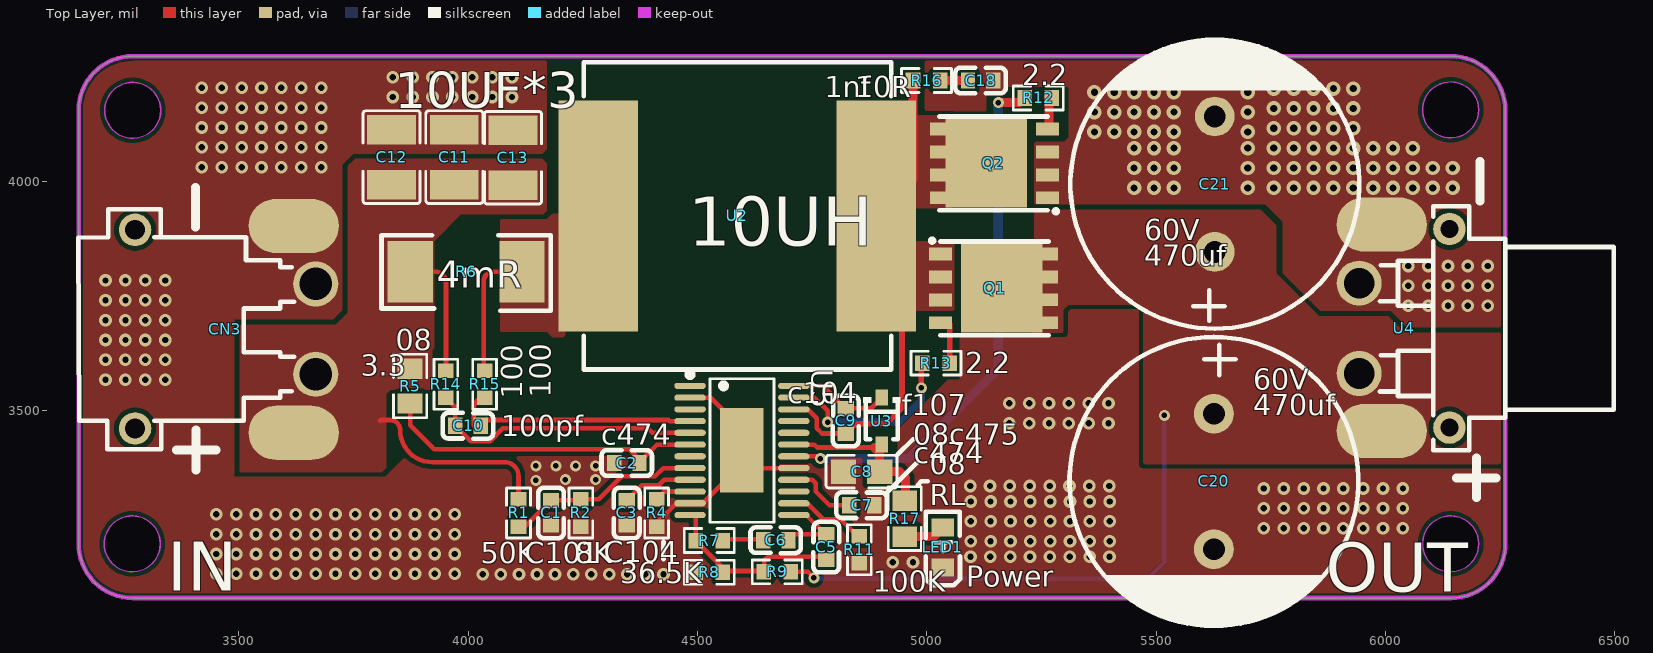
[diagram p0: Top Layer view]
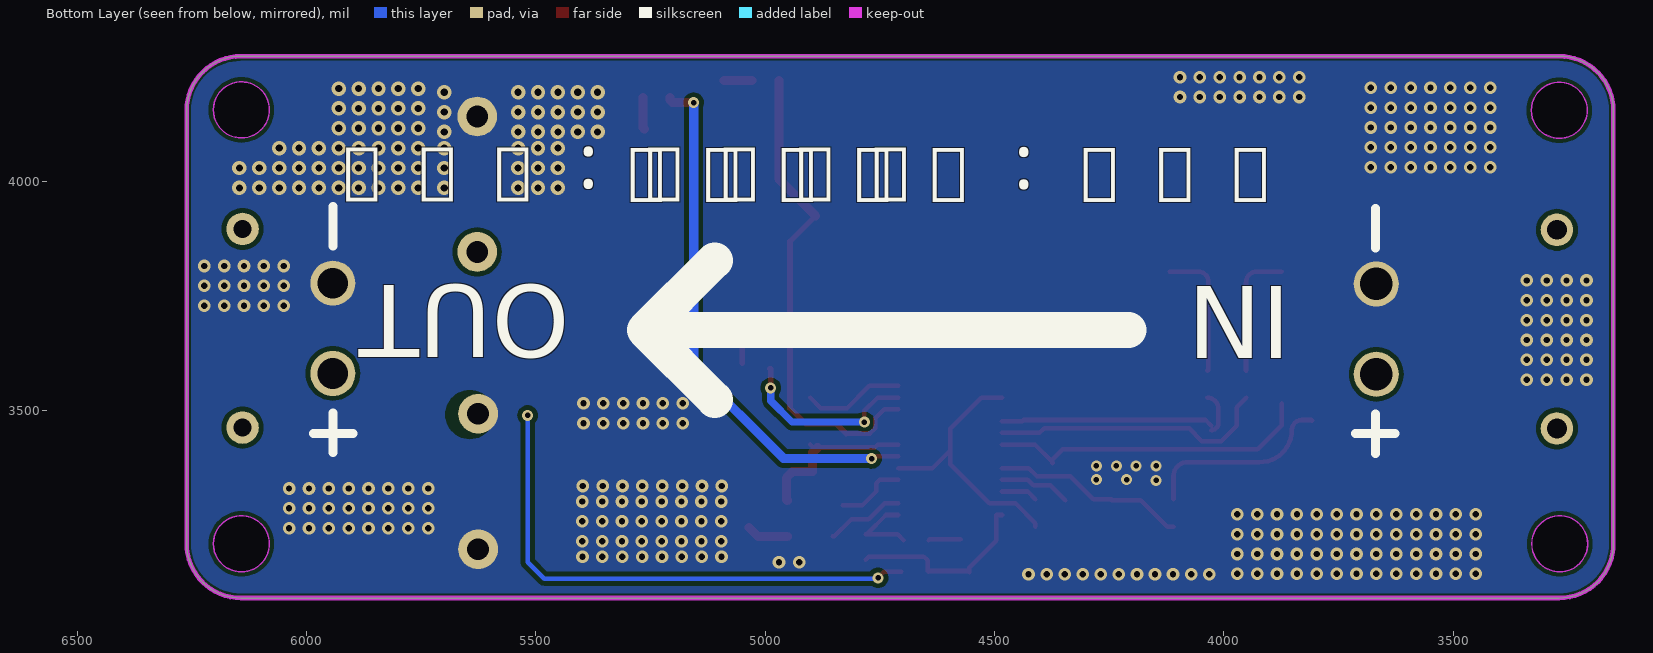
[diagram p1: Bottom Layer view, seen from below]
# Altium PCB MISC52028.pcbdoc
Units mil, origin at the board's own origin, x right, y up, seen from the top; angles counter-clockwise.
Board outline 3110.24 x 1181.1 mil, 2 copper layers (Top Layer, Bottom Layer), stack 62.206 mil thick; 38 components, 24 nets, 121 pads, 315 vias.

## Layer stack, top to bottom
Top Solder Mask Layer: solder mask 0.394, Dk 3.3
Top Layer: signal copper 1.379
Dielectric1: surface 59.449, FR4, Dk 4.5
Bottom Layer: signal copper 1.378
Bottom Solder Mask Layer: solder mask 0.394, Dk 3.3

## Board outline
3269.11,4273 ccw(c3269.11,4154.89) 3151,4154.89 3151,3210.01 ccw(c3269.11,3210.01) 3269.11,3091.9 6143.13,3091.9 ccw(c6143.13,3210.01) 6261.24,3210.01 6261.24,4154.89 ccw(c6143.13,4154.89) 6143.13,4273
cut-out: 3330.02,4155 cw(c3269,4155) 3207.98,4155 cw(c3269,4155)
cut-out: 6203.02,4156 cw(c6142,4156) 6080.98,4156 cw(c6142,4156)
cut-out: 6203.02,3210 cw(c6142,3210) 6080.98,3210 cw(c6142,3210)
cut-out: 3329.02,3210 cw(c3268,3210) 3206.98,3210 cw(c3268,3210)

## Design rules (kind name [scope] priority, off if disabled: settings)
BoardOutlineClearance copperThickness2oz_1 [All] p2 off: genericclearance=7.99 ignorepadtopadclearanceinfootprint=FALSE except(0: Arc-SplitContinuation Track-SplitContinuation SMDPad-SplitContinuation THPad-SplitContinuation Via-SplitContinuation Fill-SplitContinuation Region-SplitContinuation Poly-SplitContinuation Text-SplitContinuation Hole-SplitContinuation; 5.98: SMDPad-CutoutEdge THPad-CutoutEdge Via-CutoutEdge Fill-CutoutEdge Region-CutoutEdge Text-CutoutEdge Hole-CutoutEdge; 10: Poly-OutlineEdge Poly-CutoutEdge; 11.81: Arc-OutlineEdge Track-OutlineEdge SMDPad-OutlineEdge THPad-OutlineEdge Via-OutlineEdge Fill-OutlineEdge Region-OutlineEdge Text-OutlineEdge Hole-OutlineEdge Arc-CutoutEdge Track-CutoutEdge)
BoardOutlineClearance Plane_innerPlane_1 [All] p4 off: genericclearance=4.02 ignorepadtopadclearanceinfootprint=FALSE except(0: Arc-SplitContinuation Track-SplitContinuation SMDPad-SplitContinuation THPad-SplitContinuation Via-SplitContinuation Fill-SplitContinuation Region-SplitContinuation Poly-SplitContinuation Text-SplitContinuation Hole-SplitContinuation; 5.98: SMDPad-CutoutEdge THPad-CutoutEdge Via-CutoutEdge Fill-CutoutEdge Region-CutoutEdge Text-CutoutEdge Hole-CutoutEdge; 10: Poly-OutlineEdge Poly-CutoutEdge; 11.81: Arc-OutlineEdge Track-OutlineEdge SMDPad-OutlineEdge THPad-OutlineEdge Via-OutlineEdge Fill-OutlineEdge Region-OutlineEdge Text-OutlineEdge Hole-OutlineEdge Arc-CutoutEdge Track-CutoutEdge)
BoardOutlineClearance Copper_copperRegion_1 [All] p6 off: genericclearance=4.02 ignorepadtopadclearanceinfootprint=FALSE except(0: Arc-SplitContinuation Track-SplitContinuation SMDPad-SplitContinuation THPad-SplitContinuation Via-SplitContinuation Fill-SplitContinuation Region-SplitContinuation Poly-SplitContinuation Text-SplitContinuation Hole-SplitContinuation; 5.98: SMDPad-CutoutEdge THPad-CutoutEdge Via-CutoutEdge Fill-CutoutEdge Region-CutoutEdge Text-CutoutEdge Hole-CutoutEdge; 10: Poly-OutlineEdge Poly-CutoutEdge; 11.81: Arc-OutlineEdge Track-OutlineEdge SMDPad-OutlineEdge THPad-OutlineEdge Via-OutlineEdge Fill-OutlineEdge Region-OutlineEdge Text-OutlineEdge Hole-OutlineEdge Arc-CutoutEdge Track-CutoutEdge)
BoardOutlineClearance Copper_全直连_1 [All] p8 off: genericclearance=4.02 ignorepadtopadclearanceinfootprint=FALSE except(0: Arc-SplitContinuation Track-SplitContinuation SMDPad-SplitContinuation THPad-SplitContinuation Via-SplitContinuation Fill-SplitContinuation Region-SplitContinuation Poly-SplitContinuation Text-SplitContinuation Hole-SplitContinuation; 5.98: SMDPad-CutoutEdge THPad-CutoutEdge Via-CutoutEdge Fill-CutoutEdge Region-CutoutEdge Text-CutoutEdge Hole-CutoutEdge; 10: Poly-OutlineEdge Poly-CutoutEdge; 11.81: Arc-OutlineEdge Track-OutlineEdge SMDPad-OutlineEdge THPad-OutlineEdge Via-OutlineEdge Fill-OutlineEdge Region-OutlineEdge Text-OutlineEdge Hole-OutlineEdge Arc-CutoutEdge Track-CutoutEdge)
BoardOutlineClearance Copper_copperRegion2_1 [All] p10 off: genericclearance=4.02 ignorepadtopadclearanceinfootprint=FALSE except(0: Arc-SplitContinuation Track-SplitContinuation SMDPad-SplitContinuation THPad-SplitContinuation Via-SplitContinuation Fill-SplitContinuation Region-SplitContinuation Poly-SplitContinuation Text-SplitContinuation Hole-SplitContinuation; 5.98: SMDPad-CutoutEdge THPad-CutoutEdge Via-CutoutEdge Fill-CutoutEdge Region-CutoutEdge Text-CutoutEdge Hole-CutoutEdge; 10: Poly-OutlineEdge Poly-CutoutEdge; 11.81: Arc-OutlineEdge Track-OutlineEdge SMDPad-OutlineEdge THPad-OutlineEdge Via-OutlineEdge Fill-OutlineEdge Region-OutlineEdge Text-OutlineEdge Hole-OutlineEdge Arc-CutoutEdge Track-CutoutEdge)
BoardOutlineClearance copperThickness1oz_1 [All] p12: genericclearance=4.02 ignorepadtopadclearanceinfootprint=FALSE except(0: Arc-SplitContinuation Track-SplitContinuation SMDPad-SplitContinuation THPad-SplitContinuation Via-SplitContinuation Fill-SplitContinuation Region-SplitContinuation Poly-SplitContinuation Text-SplitContinuation Hole-SplitContinuation; 5.98: SMDPad-CutoutEdge THPad-CutoutEdge Via-CutoutEdge Fill-CutoutEdge Region-CutoutEdge Text-CutoutEdge Hole-CutoutEdge; 10: Poly-OutlineEdge Poly-CutoutEdge; 11.81: Arc-OutlineEdge Track-OutlineEdge SMDPad-OutlineEdge THPad-OutlineEdge Via-OutlineEdge Fill-OutlineEdge Region-OutlineEdge Text-OutlineEdge Hole-OutlineEdge Arc-CutoutEdge Track-CutoutEdge)
Clearance copperThickness2oz [All] p1 off: gap=7.99 ignorepadtopadclearanceinfootprint=FALSE except(5.98: SMDPad-Track SMDPad-SMDPad THPad-Track SMDPad-THPad THPad-THPad Track-Via SMDPad-Via THPad-Via Via-Via Fill-Track Region-Track Fill-SMDPad Region-SMDPad Fill-THPad Region-THPad Fill-Via Region-Via Fill-Fill Fill-Region Region-Region Arc-Track Arc-SMDPad Arc-THPad Arc-Via Fill-Arc Region-Arc Arc-Arc Text-Track SMDPad-Text Text-THPad Text-Via Fill-Text Region-Text Arc-Text Text-Text Hole-Track Hole-SMDPad Hole-THPad Hole-Via Fill-Hole Region-Hole Hole-Arc Hole-Text; 10: Poly-Track Poly-SMDPad Poly-THPad Poly-Via Poly-Fill Poly-Region Poly-Poly Poly-Arc Poly-Text Poly-Hole)
Clearance Plane_innerPlane [All] p3 off: gap=4.02 ignorepadtopadclearanceinfootprint=FALSE except(5.98: SMDPad-Track SMDPad-SMDPad THPad-Track SMDPad-THPad THPad-THPad Track-Via SMDPad-Via THPad-Via Via-Via Fill-Track Region-Track Fill-SMDPad Region-SMDPad Fill-THPad Region-THPad Fill-Via Region-Via Fill-Fill Fill-Region Region-Region Arc-Track Arc-SMDPad Arc-THPad Arc-Via Fill-Arc Region-Arc Arc-Arc Text-Track SMDPad-Text Text-THPad Text-Via Fill-Text Region-Text Arc-Text Text-Text Hole-Track Hole-SMDPad Hole-THPad Hole-Via Fill-Hole Region-Hole Hole-Arc Hole-Text; 10: Poly-Track Poly-SMDPad Poly-THPad Poly-Via Poly-Fill Poly-Region Poly-Poly Poly-Arc Poly-Text Poly-Hole)
Clearance Copper_copperRegion [All] p5 off: gap=4.02 ignorepadtopadclearanceinfootprint=FALSE except(5.98: SMDPad-Track SMDPad-SMDPad THPad-Track SMDPad-THPad THPad-THPad Track-Via SMDPad-Via THPad-Via Via-Via Fill-Track Region-Track Fill-SMDPad Region-SMDPad Fill-THPad Region-THPad Fill-Via Region-Via Fill-Fill Fill-Region Region-Region Arc-Track Arc-SMDPad Arc-THPad Arc-Via Fill-Arc Region-Arc Arc-Arc Text-Track SMDPad-Text Text-THPad Text-Via Fill-Text Region-Text Arc-Text Text-Text Hole-Track Hole-SMDPad Hole-THPad Hole-Via Fill-Hole Region-Hole Hole-Arc Hole-Text; 10: Poly-Track Poly-SMDPad Poly-THPad Poly-Via Poly-Fill Poly-Region Poly-Poly Poly-Arc Poly-Text Poly-Hole)
Clearance Copper_全直连 [All] p7 off: gap=4.02 ignorepadtopadclearanceinfootprint=FALSE except(5.98: SMDPad-Track SMDPad-SMDPad THPad-Track SMDPad-THPad THPad-THPad Track-Via SMDPad-Via THPad-Via Via-Via Fill-Track Region-Track Fill-SMDPad Region-SMDPad Fill-THPad Region-THPad Fill-Via Region-Via Fill-Fill Fill-Region Region-Region Arc-Track Arc-SMDPad Arc-THPad Arc-Via Fill-Arc Region-Arc Arc-Arc Text-Track SMDPad-Text Text-THPad Text-Via Fill-Text Region-Text Arc-Text Text-Text Hole-Track Hole-SMDPad Hole-THPad Hole-Via Fill-Hole Region-Hole Hole-Arc Hole-Text; 10: Poly-Track Poly-SMDPad Poly-THPad Poly-Via Poly-Fill Poly-Region Poly-Poly Poly-Arc Poly-Text Poly-Hole)
Clearance Copper_copperRegion2 [All] p9 off: gap=4.02 ignorepadtopadclearanceinfootprint=FALSE except(5.98: SMDPad-Track SMDPad-SMDPad THPad-Track SMDPad-THPad THPad-THPad Track-Via SMDPad-Via THPad-Via Via-Via Fill-Track Region-Track Fill-SMDPad Region-SMDPad Fill-THPad Region-THPad Fill-Via Region-Via Fill-Fill Fill-Region Region-Region Arc-Track Arc-SMDPad Arc-THPad Arc-Via Fill-Arc Region-Arc Arc-Arc Text-Track SMDPad-Text Text-THPad Text-Via Fill-Text Region-Text Arc-Text Text-Text Hole-Track Hole-SMDPad Hole-THPad Hole-Via Fill-Hole Region-Hole Hole-Arc Hole-Text; 10: Poly-Track Poly-SMDPad Poly-THPad Poly-Via Poly-Fill Poly-Region Poly-Poly Poly-Arc Poly-Text Poly-Hole)
Clearance copperThickness1oz [All] p11: gap=4.02 ignorepadtopadclearanceinfootprint=FALSE except(5.98: SMDPad-Track SMDPad-SMDPad THPad-Track SMDPad-THPad THPad-THPad Track-Via SMDPad-Via THPad-Via Via-Via Fill-Track Region-Track Fill-SMDPad Region-SMDPad Fill-THPad Region-THPad Fill-Via Region-Via Fill-Fill Fill-Region Region-Region Arc-Track Arc-SMDPad Arc-THPad Arc-Via Fill-Arc Region-Arc Arc-Arc Text-Track SMDPad-Text Text-THPad Text-Via Fill-Text Region-Text Arc-Text Text-Text Hole-Track Hole-SMDPad Hole-THPad Hole-Via Fill-Hole Region-Hole Hole-Arc Hole-Text; 10: Poly-Track Poly-SMDPad Poly-THPad Poly-Via Poly-Fill Poly-Region Poly-Poly Poly-Arc Poly-Text Poly-Hole)
DiffPairsRouting differentialPair [All] p1: maxlimit=6 minlimit=6 mostfreqgap=6 toplayer_minwidth=5 toplayer_prefwidth=10 toplayer_maxwidth=100 toplayer_mingap=6 toplayer_prefgap=6 toplayer_maxgap=6 bottomlayer_minwidth=5 bottomlayer_prefwidth=10 bottomlayer_maxwidth=100 bottomlayer_mingap=6 bottomlayer_prefgap=6 bottomlayer_maxgap=6 maxuncoupledlength=10
HoleToHoleClearance otherClearance [All] p1: gap=11.8 allowstackedmicrovias=TRUE
Length netLength [All] p1: minlimit=0 maxlimit=0
PasteMaskExpansion pasteMaskExpansion [All] p1: expansion=0
PlaneConnect innerPlane [All] p1: planeconnectstyle=Relief reliefexpansion=20 reliefentries=4 reliefconductorwidth=10 reliefairgap=10
PolygonConnect 全直连 [All] p1 off: connectstyle=Direct reliefconductorwidth=10 reliefentries=4 polygonreliefangle="90 Angle" airgapwidth=10 via.connectstyle=Relief via.reliefconductorwidth=10 via.reliefentries=4 via.polygonreliefangle="90 Angle" via.airgapwidth=10
PolygonConnect copperRegion2 [All] p2 off: connectstyle=Relief reliefconductorwidth=10 reliefentries=4 polygonreliefangle="90 Angle" airgapwidth=10 via.connectstyle=Relief via.reliefconductorwidth=10 via.reliefentries=4 via.polygonreliefangle="90 Angle" via.airgapwidth=10
PolygonConnect copperRegion [All] p3: connectstyle=Relief reliefconductorwidth=10 reliefentries=4 polygonreliefangle="90 Angle" airgapwidth=10 via.connectstyle=Relief via.reliefconductorwidth=10 via.reliefentries=4 via.polygonreliefangle="90 Angle" via.airgapwidth=10
RoutingVias viaSize [All] p1: holewidth=12.01 width=24.02 viastyle="Through Hole" minholewidth=11.81 minwidth=19.68 maxholewidth=248.03 maxwidth=393.7
SolderMaskExpansion solderMaskExpansion [IsVia] p1: expansion=-1000 istentingtop=TRUE
SolderMaskExpansion solderMaskExpansion [All] p2: expansion=2.01 istentingtop=FALSE
Width copperThickness2oz_2 [All] p1 off: maxlimit=100 minlimit=8 preferedwidth=10
Width copperThickness1oz_2 [All] p2: maxlimit=100 minlimit=5 preferedwidth=10

## Components (designator, comment, footprint, x,y, rotation, side; value= is the part's Value field where it differs from the comment)
C1 "100pF" C0603 4181,3277.61 r90 top
C2 "470nF" C0603 4346.2,3386.16 r0 top
C3 "100nF" C0603 4346,3277.61 r90 top
C5 "300pF" C0603 4781,3203 r90 top
C6 "34nF" C0603 4671,3217.84 r0 top
C7 "470nF" C0603 4858.16,3294 r0 top
C8 "4.7uf" C0805 4857.86,3367.46 r180 top
C9 "100nF" C0603 4823.65,3478 r90 top
C10 "100pf" C0603 4000,3467.3 r0 top
C11 "10uF" C1210 3970.17,4053 r270 top
C12 "10uF" C1210 3833.24,4053 r270 top
C13 "10uF" C1210 4097.93,4051.73 r270 top
C18 "100nF" C0603 5117.5,4220 r0 top
C20 "470uF" CAP-TH_BD16.0-P7.50-D1.2-FD 5626,3346 r270 top
C21 "470uF" CAP-TH_BD16.0-P7.50-D1.2-FD 5628,3994 r90 top
CN3 "XT30PW-M" CONN-TH_XT30PW-M 3471,3678 r270 top
LED1 "" LED_0805 5035.33,3204 r90 top
Q1 "CSD18540Q5B" VSON-CLIP-8_L5.0-W6.0-P1.27-BL 5147.91,3766.73 r270 top
Q2 "CSD18540Q5B" VSON-CLIP-8_L5.0-W6.0-P1.27-BL 5145.16,4039.22 r90 top
R1 "50K" R0603 4110,3277.31 r90 top
R2 "8K" R0603 4246,3277.31 r90 top
R4 "36.5K" R0603 4411,3277.31 r90 top
R5 "3.3" R0805_NEW 3873.84,3554 r90 top
R6 "4mΩ" RES-SMD_L6.4-W3.2-1 3995.89,3803 r0 top
R7 "40.53K" R0603 4526,3217.13 r0 top
R8 "1.6K" R0603 4526,3148 r0 top
R9 "30K" R0603 4673.84,3148.98 r0 top
R11 "100K" R0603 4852.97,3197.04 r90 top
R12 "2.2" R0603 5243.24,4182 r0 top
R13 "10K" R0603 5020,3604 r0 top
R14 "100" R0603 3951.66,3558 r90 top
R15 "100" R0603 4036,3558 r90 top
R16 "10K" R0603 4999.63,4220 r0 top
R17 "10K" R0805 4952,3265 r90 top
U2 "10uH" IND-SMD_L17.0-W17.0_YSPIA1770-100M 4587.2,3925 r0 top
U3 "FR107WS" SOD-323_L1.6-W1.3-LS2.7-RD 4902,3477.7 r270 top
U4 "XT30PW-F" CONN-TH_XT30PW-F-1 6041,3679.85 r90 top
U5 "LM5122ZAPWPR" HTSSOP-24_L7.8-W4.4-P0.65-LS6.4-BL-EP-3 4597.03,3413.55 r270 top

## Footprints (in the part's own frame and the unit in brackets; to place one, negate y for a bottom-side part, rotate by r counter-clockwise, add the part's x,y. Pads: shape width x height; smd on the part's side, far side on the other; paste and mask are expansions set on the pad)
C0603 [mm]
  rect 0.8x0.9 smd: 1(-0.7,0) 2(0.7,0)
  silkscreen extent -1.41,-0.71 1.39,0.72
C0805 [mm]
  rect 1.41x1.35 smd paste-100 mask+0.051: 1(-1,0) 2(1,0)
  silkscreen extent -1.96,-0.9 1.96,0.9
C1210 [mm]
  rect 1.635x2.7 smd paste-100 mask+0.051: 1(-1.517,0) 2(1.517,0)
  silkscreen extent -2.56,-1.58 2.56,1.58
CAP-TH_BD16.0-P7.50-D1.2-FD [mm]
  round 2.2 hole 1.2: 1(-3.75,0) 2(3.75,0)
  silkscreen extent -8,-8 8,8
CONN-TH_XT30PW-F-1 [mm]
  round 2.5 hole 1.7 copper offset 0,0: 1(-2.5,2.5) 2(2.5,2.5)
  round 1.8 hole 1 copper offset 0,0: 3(5.5,-2.5) 4(-5.5,-2.5)
  silkscreen extent -6.75,-11.6 6.75,1.35
CONN-TH_XT30PW-M [mm]
  round 2.5 hole 1.8: 1(-2.5,5) 2(2.5,5)
  round 1.8 hole 1.1: 3(5.5,-5) 4(-5.5,-5)
  silkscreen extent -6.65,-8.15 6.65,3.81
HTSSOP-24_L7.8-W4.4-P0.65-LS6.4-BL-EP-3 [mm]
  oval 0.343x1.747 smd: 1(-3.575,-2.873) 2(-2.925,-2.873) 3(-2.275,-2.873) 4(-1.625,-2.873) 5(-0.975,-2.873) 6(-0.325,-2.873) 7(0.325,-2.873) 8(0.975,-2.873) 9(1.625,-2.873) 10(2.275,-2.873) 11(2.925,-2.873) 12(3.575,-2.873) 13(3.575,2.873) 14(2.925,2.873) 15(2.275,2.873) 16(1.625,2.873) 17(0.975,2.873) 18(0.325,2.873) 19(-0.325,2.873) 20(-0.975,2.873) 21(-1.625,2.873) 22(-2.275,2.873) 23(-2.925,2.873) 24(-3.575,2.873)
  rect 4.68x2.4 smd: 25(0,0)
  silkscreen extent -4.35,-3.02 3.98,1.77
IND-SMD_L17.0-W17.0_YSPIA1770-100M [mm]
  rect 4.4x12.8 smd paste+0 mask+0.05: 1(-7.7,0) 2(7.7,0)
  silkscreen extent -8.51,-8.51 8.51,8.51
LED_0805 [mm]
  rect 1x1.25 smd paste+0 mask+0.051: 1(-1.15,0.005) 2(1.05,0.005)
  silkscreen extent -2.15,-0.94 1.93,0.97
R0603 [mil]
  rect 31.75x34.02 smd paste-3937.01 mask+2: 1(-29.66,0) 2(29.66,0)
  silkscreen extent -55,-26 55,26
R0805 [mm]
  rect 1.133x1.377 smd paste-100 mask+0.051: 1(-1,0) 2(1,0)
  silkscreen extent -1.76,-0.92 1.76,0.92
R0805_NEW [mil]
  rect 44.59x54.21 smd paste-3937.01 mask+2: 1(-38.04,0) 2(38.04,0)
  silkscreen extent -69,-36 69,36
RES-SMD_L6.4-W3.2-1 [mm]
  rect 2.5x3.4 smd: 1(-3.1,0) 2(3.1,0)
  silkscreen extent -4.69,-2.16 4.69,2.03
SOD-323_L1.6-W1.3-LS2.7-RD [mm]
  rect 0.9x0.7 smd paste+0 mask+0.05: 1(-1.3,0) 2(1.3,0)
  silkscreen extent -1.32,-1.02 1.02,1.02
VSON-CLIP-8_L5.0-W6.0-P1.27-BL [mm]
  rect 0.7x1.27 smd paste-100 mask+0.051: 1(-1.904,-3) 2(-0.636,-3) 3(0.636,-3) 4(1.906,-3)
  rect 0.7x1 smd paste-100 mask+0.051: 5(1.904,3) 6(0.634,3) 7(-0.636,3) 8(-1.906,3)
  rect 4.9x4.5 smd paste-100 mask+0.051: 8(-0.001,0.39)
  silkscreen extent -2.75,-3.57 2.6,3

## Free pads (board coordinates)
  oval 196.85x118.11 smd: 1(3620,3451.98) 1(3620,3903) 1(5991.79,3456) 1(5991.79,3906)

## Via types
v1: diameter 27.56, hole 13.8, Top Layer to Bottom Layer, 229 vias
v2: diameter 31.5, hole 15.7, Top Layer to Bottom Layer, 73 vias
v3: diameter 24.02, hole 12, Top Layer to Bottom Layer, 13 vias

## Nets (pads, with @x,y where several pads share a name; then routed paths per layer and width w, separated by ;. In a path a pad name is that pad's centre, name@x,y a point inside that pad or via, vN(x,y) a via of type N, cw(c..) or ccw(c..) an arc to the next point about the centre after c; other vN are vias at no path point)
$1N357: C1.2 R1.1 R2.2 U5.8 | length 426.7
  Top Layer w10: R1.1 4123.48,3247.65 C1.2 4244.2,3305.17 R2.2 4284.97,3306.97 4335.46,3357.46 4407.46,3357.46 4425.16,3375.16 U5.8
$1N466: C2.2 R5.1 U5.6 | length 710.5
  Top Layer w10: R5.1 3873.84,3468.16 3926,3416 4351.59,3416 C2.2@4376.61,3390.98 ; C2.2 4373.76,3388.13 C2.2@4376.61,3390.98 ; U5.6 4411.97,3426.34 C2.2@4376.61,3390.98
$1N636: C3.2 U5.9 | length 156.3
  Top Layer w10: C3.2 4378.83,3338 4416,3338 4427.57,3349.57 U5.9
$1N687: R4.2 U5.10 | length 80
  Top Layer w10: R4.2 4428.01,3323.98 U5.10
$1N1291: C6.1 R7.2 | length 70.3
  Top Layer w10: 4574,3220 4641.28,3220 C6.1
$1N1304: C5.2 C6.2 U5.13 | length 174.1
  Top Layer w10: C6.2 4711.28,3230.56 C5.2@4779.03,3230.56 ; U5.13 4736.79,3272.8 C5.2@4779.03,3230.56 ; C5.2 C5.2@4779.03,3230.56
$1N1428: C5.1 R7.1 R8.2 R9.1 U5.12 | length 420.1
  Top Layer w10: U5.12 4496.34,3272.8 R7.1 4555.66,3157.81 R8.2 4558.46,3150.8 R9.1@4646,3150.8 ; R9.1 R9.1@4646,3150.8 ; C5.1 4774.44,3182 4654,3182 4646,3174 R9.1@4646,3150.8
$1N1901: C9.2 U3.1 U5.24 | length 221.7
  Top Layer w10: U5.24 4772.94,3554.3 4821.68,3505.56 C9.2 4878.69,3505.56 U3.1
$1N2307: C7.1 U5.16 | length 154
  Top Layer w10: U5.16 4750.43,3349.57 4758,3342 4758,3324 4788,3294 C7.1
$1N2318: R11.2 U5.14 | length 172.5
  Top Layer w10: U5.14 4739.61,3298.39 4774,3264 4812,3264 4849.3,3226.7 R11.2
$1N3000: C9.1 Q1.1 Q1.2 Q1.3 Q2.5 Q2.6 Q2.7 Q2.8 R16.1 U2.2 U5.22 | length 1063.6
  Top Layer w10: U5.22 4740.88,3503.12 4760,3484 4760,3462 4771.56,3450.44 C9.1
  Top Layer w12: C9.1 4845.21,3472 4912,3472 4946,3506 4946,3869.34 U2.2
  Top Layer w20: U2.2 4969.97,4004.63 R16.1
$1N3130: R12.1 U5.18 | length 1168.3
  Top Layer w10: U5.18 4763.25,3400.75 v3(4768,3396)
  Top Layer w20: v3(5156,4172) 5202,4172 5207.45,4177.45 R12.1@5207.45,4183
  Bottom Layer w20: v3(4768,3396) 4960,3396 5156,3592 v3(5156,4172)
$1N3135: Q2.4 R12.2 | length 70.2
  Top Layer w20: Q2.4 5266.77,4117.75 R12.2@5266.77,4183
$1N3140: R13.1 U5.23 | length 405.8
  Top Layer w10: U5.23 4755.29,3528.71 4784,3500 v3(4784,3475.57)
  Top Layer w11.81: v3(4988,3550) 4988,3592.01 R13.1@4990.34,3592.01
  Bottom Layer w15.75: v3(4784,3475.57) 4941.57,3475.57 4988,3522 v3(4988,3550)
$1N3174: Q1.4 R13.2 | length 105.6
  Top Layer w11.81: Q1.4 5046.31,3691.69 5049.66,3688.34 R13.2
$1N3562: C10.1 R14.1 U5.5 | length 610.7
  Top Layer w10: R14.1 3972.44,3507.56 C10.1 4005.74,3434 4048,3434 4076,3462 4392,3462 4402.06,3451.94 U5.5
$1N3570: C10.2 R15.1 U5.4 | length 555.7
  Top Layer w10: C10.2 4040.26,3480 4437.06,3480 4439.53,3477.53 U5.4 ; C10.2@4027.89,3458 cw(c4027.89,3473.89) 4012,3473.89 4012,3504.34 cw(c4036,3504.34) R15.1
$1N3575: R6.2 R15.2 U2.1 | length 291.4
  Top Layer w10: R15.2 cw(c4036,3589.66) 4034,3589.66 4034,3782 cw(c4055,3782) 4055,3803 R6.2
$1N5355: C18.1 R16.2 | length 60.6
  Top Layer w20: R16.2 C18.1
$1N5615: LED1.2 R17.1 | length 91.3
  Top Layer w19.68: R17.1 5015.42,3225.63 LED1.2
AGND: C1.1 C2.1 C3.1 C7.2 C8.2 C11.1 C12.1 C13.1 C18.2 C20.2 C21.2 CN3.1 LED1.1 pad.1@3620,3903 pad.1@5991.79,3906 Q2.1 Q2.2 Q2.3 R2.1 R4.1 R8.1 R11.1 U4.2 U5.2 U5.11 U5.17 U5.25 | length 594.1
  Top Layer w10: R4.1 4411,3255 4454.39,3298.39 U5.11 4511.53,3298.39 4597.03,3383.88 U5.25 ; U5.2 4529.29,3528.71 4597.03,3460.97 U5.25 ; U5.17 4635.42,3375.16 U5.25
  other v1: 4032.22,3144 4071.59,3144 4110.96,3144 4150.33,3144 4189.7,3144 4229.07,3144 4268.44,3144 4307.81,3144 4347.18,3144 4386.55,3144 4425.92,3144 3451.16,3144.56 3494.47,3144.56 3537.78,3144.56 3581.09,3144.56 3624.39,3144.56 3667.7,3144.56 3711.01,3144.56 3754.31,3144.56 3797.62,3144.56 3840.93,3144.56 3884.24,3144.56 3927.54,3144.56 3970.85,3144.56 4926,3170 4970,3170 5095.23,3182 5138.54,3182 5181.84,3182 5225.15,3182 5268.46,3182 5311.76,3182 5355.07,3182 5398.38,3182 3451.16,3187.86 3494.47,3187.86 3537.78,3187.86 3581.09,3187.86 3624.39,3187.86 3667.7,3187.86 3711.01,3187.86 3754.31,3187.86 3797.62,3187.86 3840.93,3187.86 3884.24,3187.86 3927.54,3187.86 3970.85,3187.86 5095.78,3215.61 5139.09,3215.61 5182.39,3215.61 5225.7,3215.61 5269.01,3215.61 5312.31,3215.61 5355.62,3215.61 5398.93,3215.61 3451.16,3231.17 3494.47,3231.17 3537.78,3231.17 3581.09,3231.17 3624.39,3231.17 3667.7,3231.17 3711.01,3231.17 3754.31,3231.17 3797.62,3231.17 3840.93,3231.17 3884.24,3231.17 3927.54,3231.17 3970.85,3231.17 5734.85,3244 5778.16,3244 5821.46,3244 5864.77,3244 5908.08,3244 5951.39,3244 5994.69,3244 6038,3244 5095.78,3258.91 5139.09,3258.91 5182.39,3258.91 5225.7,3258.91 5269.01,3258.91 5312.31,3258.91 5355.62,3258.91 5398.93,3258.91 3451.16,3274.48 3494.47,3274.48 3537.78,3274.48 3581.09,3274.48 3624.39,3274.48 3667.7,3274.48 3711.01,3274.48 3754.31,3274.48 3797.62,3274.48 3840.93,3274.48 3884.24,3274.48 3927.54,3274.48 3970.85,3274.48 5734.85,3287.31 5778.16,3287.31 5821.46,3287.31 5864.77,3287.31 5908.08,3287.31 5951.39,3287.31 5994.69,3287.31 6038,3287.31 5095.78,3302.22 5139.09,3302.22 5182.39,3302.22 5225.7,3302.22 5269.01,3302.22 5312.31,3302.22 5355.62,3302.22 5398.93,3302.22 5734.85,3330.61 5778.16,3330.61 5821.46,3330.61 5864.77,3330.61 5908.08,3330.61 5951.39,3330.61 5994.69,3330.61 6038,3330.61 5094.61,3336 5137.92,3336 5181.23,3336 5224.54,3336 5267.84,3336 5311.15,3336 5354.46,3336 5397.76,3336 5179.78,3472.91 5223.09,3472.91 5266.39,3472.91 5309.7,3472.91 5353.01,3472.91 5396.31,3472.91 5179.78,3516.22 5223.09,3516.22 5266.39,3516.22 5309.7,3516.22 5353.01,3516.22 5396.31,3516.22 3209.78,3567.68 3253.09,3567.68 3296.39,3567.68 3339.7,3567.68 3209.78,3610.99 3253.09,3610.99 3296.39,3610.99 3339.7,3610.99 3209.78,3654.3 3253.09,3654.3 3296.39,3654.3 3339.7,3654.3 3209.78,3697.61 3253.09,3697.61 3296.39,3697.61 3339.7,3697.61 6049.75,3729.06 6093.06,3729.06 6136.37,3729.06 6179.67,3729.06 6222.98,3729.06 3209.78,3740.91 3253.09,3740.91 3296.39,3740.91 3339.7,3740.91 6049.75,3772.37 6093.06,3772.37 6136.37,3772.37 6179.67,3772.37 6222.98,3772.37 3209.78,3784.22 3253.09,3784.22 3296.39,3784.22 3339.7,3784.22 6049.75,3815.68 6093.06,3815.68 6136.37,3815.68 6179.67,3815.68 6222.98,3815.68 3419.78,4030.99 3463.09,4030.99 3506.39,4030.99 3549.7,4030.99 3593.01,4030.99 3636.32,4030.99 3679.62,4030.99 3419.78,4074.3 3463.09,4074.3 3506.39,4074.3 3549.7,4074.3 3593.01,4074.3 3636.32,4074.3 3679.62,4074.3 3419.78,4117.61 3463.09,4117.61 3506.39,4117.61 3549.7,4117.61 3593.01,4117.61 3636.32,4117.61 3679.62,4117.61 3419.78,4160.91 3463.09,4160.91 3506.39,4160.91 3549.7,4160.91 3593.01,4160.91 3636.32,4160.91 3679.62,4160.91 3836,4184 3879.31,4184 3922.61,4184 3965.92,4184 4009.23,4184 4052.54,4184 4095.84,4184 3419.78,4204.22 3463.09,4204.22 3506.39,4204.22 3549.7,4204.22 3593.01,4204.22 3636.32,4204.22 3679.62,4204.22 3836,4227.31 3879.31,4227.31 3922.61,4227.31 3965.92,4227.31 4009.23,4227.31 4052.54,4227.31 4095.84,4227.31
  other v2: 5452.08,3986 5495.39,3986 5538.69,3986 5699.82,3986 5756.49,3986 5799.8,3986 5843.11,3986 5886.41,3986 5929.72,3986 5973.03,3986 6016.33,3986 6059.64,3986 6102.95,3986 6146.26,3986 5452.08,4029.31 5495.39,4029.31 5538.69,4029.31 5699.82,4029.31 5756.49,4029.31 5799.8,4029.31 5843.11,4029.31 5886.41,4029.31 5929.72,4029.31 5973.03,4029.31 6016.33,4029.31 6059.64,4029.31 6102.95,4029.31 6146.26,4029.31 5452.08,4072.61 5495.39,4072.61 5538.69,4072.61 5699.82,4072.61 5756.49,4072.61 5799.8,4072.61 5843.11,4072.61 5886.41,4072.61 5929.72,4072.61 5973.03,4072.61 6016.33,4072.61 6059.64,4072.61 5365.46,4108 5408.77,4108 5452.08,4108 5495.39,4108 5538.69,4108 5699.82,4108 5756.49,4115.92 5799.8,4115.92 5843.11,4115.92 5886.41,4115.92 5929.72,4115.92 5365.46,4151.31 5408.77,4151.31 5452.08,4151.31 5495.39,4151.31 5538.69,4151.31 5699.82,4151.31 5756.49,4159.23 5799.8,4159.23 5843.11,4159.23 5886.41,4159.23 5929.72,4159.23 5365.46,4194.61 5408.77,4194.61 5452.08,4194.61 5495.39,4194.61 5538.69,4194.61 5699.82,4194.61 5756.49,4202.54 5799.8,4202.54 5843.11,4202.54 5886.41,4202.54 5929.72,4202.54
  other v3: 4148,3348.5 4212,3350 4278,3350 4148,3380 4191.31,3380 4234.61,3380 4277.92,3380
VCC: C8.1 R17.2 U3.2 U5.19 | length 367.2
  Top Layer w10: U5.19 4754.53,3426.34 4760.87,3420 4886,3420 4895.48,3420 U3.2
  Top Layer w19.68: 4886,3420 4897.23,3408.77 C8.1 4940.54,3367.46 4954,3354 4954,3306.37 R17.2
VIN: C11.2 C12.2 C13.2 CN3.2 pad.1@3620,3451.98 R1.2 R5.2 R6.1 R14.2 | length 707.6
  Top Layer w10: 3808,3478 cw(c3810,3478) 3810,3480 3830,3480 cw(c3830,3458) 3852,3458 ccw(c3922,3458) 3922,3388 4080,3388 cw(c4080,3358) 4110,3358 R1.2 ; R6.1 3929,3803 cw(c3929,3780) 3952,3780 3952,3588 cw(c3951.66,3588) R14.2
VOUT: C20.1 C21.1 pad.1@5991.79,3456 Q1.5 Q1.6 Q1.7 Q1.8 R9.2 U4.1 | length 1155.6
  Top Layer w10: R9.2 4741.02,3148.98 v3(4754,3136)
  Bottom Layer w10: v3(4754,3136) 4756,3134 5482,3134 5518,3170 v3(5518,3490)
pads on no net: CN3.3 CN3.4 U4.3 U4.4 U5.1 U5.3 U5.7 U5.15 U5.20 U5.21

## Polygon pours and split planes (outlines as drawn)
AGND on Top Layer (solid, remove dead copper, pour order 0): 3106,4492 4172,4492 4172,4070 4162,4060 3750,4060 3726,4036 3726,3719.55 3706,3699.55 3106,3699.55
VIN on Top Layer (solid, remove dead copper, pour order 2): 3502,3688 3712,3688 3738,3714 3738,4034 3754,4050 4162,4050 4172,4040 4172,3936.15 4164,3928.15 3984.15,3928.15 3926,3870 3926,3636 3922,3632 3922,3550 3918,3546 3832,3546 3822,3536 3822,3376 3812,3366 3502,3366
$1N3575 on Top Layer (solid, remove dead copper, pour order 4): 4070,3918 4172,3918 4184,3930 4212,3930 4212,3664.73 4208,3660.73 4183.27,3660.73 4172,3672 4070,3672
$1N3000 on Top Layer (solid, remove dead copper, pour order 6): 4822,4144 5054.25,4144 5054.25,3943.75 5056,3942 4822,3942
$1N3000 on Top Layer (solid, remove dead copper, pour order 8): 4834,3870 4834,3718 5060,3718 5060,3870
AGND on Top Layer (solid, remove dead copper, pour order 10): 5234,4086 5300,4086 5310,4096 5310,4202 5306,4206 5179.03,4206 5168.65,4195.62 5135.62,4195.62 5130,4190 5130,4152.61 4996.61,4152.61 4996,4152 4996,4302 4998,4304 6350,4304 6360,4294 6360,3682 6048,3682 6012,3718 5858,3718 5776,3800 5776,3912 5738,3950 5234,3950
VOUT on Top Layer (solid, remove dead copper, pour order 12): 5222,3670 5298,3670 5298,3719.94 5309.36,3731.3 5462.7,3731.3 5472,3722 5472,3384 6348,3384 6358,3394 6358,3670 6042,3670 6006,3706 5855.51,3706 5762,3799.51 5762,3904 5728,3938 5234,3938 5234,3752 5226,3744 5226,3674
AGND on Top Layer (solid, remove dead copper, pour order 14): 3102,3784 3398,3784 3404,3778 3488,3778 3490,3776 3490,3356 3820,3356 3870,3406 4524.61,3406 4524.61,3257.18 4677.18,3257.18 4678,3258 4678,3396.79 4935.86,3396.79 4936.65,3396 4936.65,3458.65 5046,3568 5072,3568 5072,3658 5074,3660 5298,3660 5306,3668 5306,3714 5314,3722 5458,3722 5466,3714 5466,3376 6442,3376 6480,3338 6480,3092 6388,3000 3168,3000 3092,3076 3092,3774
AGND on Bottom Layer (solid, remove dead copper, pour order 16): 3018,4332 6300,4332 6312,4344 6340,4316 6340,3050 3006,3050 3000,3056 3000,4314

## Keep-outs
Board Outline Layer:
  region: 3330.02,4155 cw(c3269,4155) 3207.98,4155 cw(c3269,4155)
  circle w0.1: c3269,4155 r61.02
  region: 3330.02,4155 3329.64,4148.17 3328.49,4141.42 3326.6,4134.85 3323.98,4128.52 3320.67,4122.53 3316.71,4116.95 3312.15,4111.85 3307.05,4107.29 3301.47,4103.33 3295.48,4100.02 3289.15,4097.4 3282.58,4095.51 3275.83,4094.36 3269,4093.98 3262.17,4094.36 3255.42,4095.51 3248.85,4097.4 3242.52,4100.02 3236.53,4103.33 3230.95,4107.29 3225.85,4111.85 3221.29,4116.95 3217.33,4122.53 3214.02,4128.52 3211.4,4134.85 3209.51,4141.42 3208.36,4148.17 3207.98,4155 3208.36,4161.83 3209.51,4168.58 3211.4,4175.15 3214.02,4181.48 3217.33,4187.47 3221.29,4193.05 3225.85,4198.15 3230.95,4202.71 3236.53,4206.67 3242.52,4209.98 3248.85,4212.6 3255.42,4214.49 3262.17,4215.64 3269,4216.02 3275.83,4215.64 3282.58,4214.49 3289.15,4212.6 3295.48,4209.98 3301.47,4206.67 3307.05,4202.71 3312.15,4198.15 3316.71,4193.05 3320.67,4187.47 3323.98,4181.48 3326.6,4175.15 3328.49,4168.58 3329.64,4161.83
  region: 6203.02,4156 cw(c6142,4156) 6080.98,4156 cw(c6142,4156)
  circle w0.1: c6142,4156 r61.02
  region: 6203.02,4156 6202.64,4149.17 6201.49,4142.42 6199.6,4135.85 6196.98,4129.52 6193.67,4123.53 6189.71,4117.95 6185.15,4112.85 6180.05,4108.29 6174.47,4104.33 6168.48,4101.02 6162.15,4098.4 6155.58,4096.51 6148.83,4095.36 6142,4094.98 6135.17,4095.36 6128.42,4096.51 6121.85,4098.4 6115.52,4101.02 6109.53,4104.33 6103.95,4108.29 6098.85,4112.85 6094.29,4117.95 6090.33,4123.53 6087.02,4129.52 6084.4,4135.85 6082.51,4142.42 6081.36,4149.17 6080.98,4156 6081.36,4162.83 6082.51,4169.58 6084.4,4176.15 6087.02,4182.48 6090.33,4188.47 6094.29,4194.05 6098.85,4199.15 6103.95,4203.71 6109.53,4207.67 6115.52,4210.98 6121.85,4213.6 6128.42,4215.49 6135.17,4216.64 6142,4217.02 6148.83,4216.64 6155.58,4215.49 6162.15,4213.6 6168.48,4210.98 6174.47,4207.67 6180.05,4203.71 6185.15,4199.15 6189.71,4194.05 6193.67,4188.47 6196.98,4182.48 6199.6,4176.15 6201.49,4169.58 6202.64,4162.83
  region: 6203.02,3210 cw(c6142,3210) 6080.98,3210 cw(c6142,3210)
  circle w0.1: c6142,3210 r61.02
  region: 6203.02,3210 6202.64,3203.17 6201.49,3196.42 6199.6,3189.85 6196.98,3183.52 6193.67,3177.53 6189.71,3171.95 6185.15,3166.85 6180.05,3162.29 6174.47,3158.33 6168.48,3155.02 6162.15,3152.4 6155.58,3150.51 6148.83,3149.36 6142,3148.98 6135.17,3149.36 6128.42,3150.51 6121.85,3152.4 6115.52,3155.02 6109.53,3158.33 6103.95,3162.29 6098.85,3166.85 6094.29,3171.95 6090.33,3177.53 6087.02,3183.52 6084.4,3189.85 6082.51,3196.42 6081.36,3203.17 6080.98,3210 6081.36,3216.83 6082.51,3223.58 6084.4,3230.15 6087.02,3236.48 6090.33,3242.47 6094.29,3248.05 6098.85,3253.15 6103.95,3257.71 6109.53,3261.67 6115.52,3264.98 6121.85,3267.6 6128.42,3269.49 6135.17,3270.64 6142,3271.02 6148.83,3270.64 6155.58,3269.49 6162.15,3267.6 6168.48,3264.98 6174.47,3261.67 6180.05,3257.71 6185.15,3253.15 6189.71,3248.05 6193.67,3242.47 6196.98,3236.48 6199.6,3230.15 6201.49,3223.58 6202.64,3216.83
  region: 3329.02,3210 cw(c3268,3210) 3206.98,3210 cw(c3268,3210)
  circle w0.1: c3268,3210 r61.02
  region: 3329.02,3210 3328.64,3203.17 3327.49,3196.42 3325.6,3189.85 3322.98,3183.52 3319.67,3177.53 3315.71,3171.95 3311.15,3166.85 3306.05,3162.29 3300.47,3158.33 3294.48,3155.02 3288.15,3152.4 3281.58,3150.51 3274.83,3149.36 3268,3148.98 3261.17,3149.36 3254.42,3150.51 3247.85,3152.4 3241.52,3155.02 3235.53,3158.33 3229.95,3162.29 3224.85,3166.85 3220.29,3171.95 3216.33,3177.53 3213.02,3183.52 3210.4,3189.85 3208.51,3196.42 3207.36,3203.17 3206.98,3210 3207.36,3216.83 3208.51,3223.58 3210.4,3230.15 3213.02,3236.48 3216.33,3242.47 3220.29,3248.05 3224.85,3253.15 3229.95,3257.71 3235.53,3261.67 3241.52,3264.98 3247.85,3267.6 3254.42,3269.49 3261.17,3270.64 3268,3271.02 3274.83,3270.64 3281.58,3269.49 3288.15,3267.6 3294.48,3264.98 3300.47,3261.67 3306.05,3257.71 3311.15,3253.15 3315.71,3248.05 3319.67,3242.47 3322.98,3236.48 3325.6,3230.15 3327.49,3223.58 3328.64,3216.83
  lines w10: 3151,3210.01 3151,4154.89 cw(c3269.11,4154.89) 3269.11,4273 6143.13,4273 cw(c6143.13,4154.89) 6261.24,4154.89 6261.24,3210.01 cw(c6143.13,3210.01) 6143.13,3091.9 3269.11,3091.9 cw(c3269.11,3210.01) 3151,3210.01

## Silkscreen, mask and mechanical layers (free items; w line width, h text height)
Top Silkscreen Layer:
  lines w10: 4426,3176 4426,3214 ; 4909.31,3318.36 4976.95,3386 4978,3386 ; 4936,3404 4970,3438 4972,3438 ; 4980,3338 4988,3346 5002,3346
  lines w19.68: 3364.24,3414.55 3450.54,3414.55 ; 3406,3900.85 3406,3987.15 ; 3407.39,3371.4 3407.39,3457.7 ; 6154.85,3354 6241.15,3354 ; 6198,3310.85 6198,3397.15 ; 6206,3956.85 6206,4043.15
  text "2.2" at 5208,4210 h45
  text "1nf" at 4778,4184 h45
  text "10R" at 4844,4184 h45
  text "10UF*3" at 3840,4160 h78.74
  text "60V" at 5474,3872 h45
  text "10UH" at 4480,3860 h106.3
  text "470uf" at 5474,3816 h45
  text "4mR" at 3932,3768 h59.06
  text "08" at 3842,3632 h45
  text "2.2" at 5084,3582 h45
  text "3.3" at 3766,3576 h45
  text "60V" at 5712,3546 h45
  text "100" at 4180,3528 h45 r90
  text "100" at 4118,3526 h45 r90
  text "c104" at 4696,3516 h45
  text "f107" at 4946,3490 h45
  text "470uf" at 5712,3490 h45
  text "100pf" at 4072,3444 h45
  text "c474" at 4290,3426 h45
  text "08c475" at 4970,3426 h45
  text "c474" at 4972,3386 h45
  text "08 / RL" at 5006,3294 h45
  text "C104" at 4296,3170 h45
  text "50K" at 4028,3168 h45
  text "C101" at 4124,3168 h45
  text "8K" at 4234,3168 h45
  text "36.5K" at 4332,3124 h45
  text "Power" at 5086,3116 h45
  text "IN" at 3344,3108 h106.3
  text "100K" at 4882,3106 h45
  text "OUT" at 5870,3106 h106.3
Bottom Silkscreen Layer:
  lines w19.68: 3626.85,3450 3713.15,3450 ; 3670,3406.85 3670,3493.15 ; 3670,3854.85 3670,3941.15 ; 5898.85,3450 5985.15,3450 ; 5942,3408.85 5942,3495.15 ; 5942,3858.85 5942,3945.15
  lines w78.74: 4208.25,3676.01 5262,3676.01 ; 5110,3524.01 5262,3676.01 ; 5110,3828.01 5262,3676.01
  text "VOUT：48V" at 4644.18,4073.64 h120 r180
  text "VIN：5~60V" at 3860.18,4072.55 h120 r180
  text "OUT" at 5426,3773.91 h157.48 r180
  text "IN" at 3854,3772 h157.48 r180
Mechanical Layer:
  circle w0.1: c3269,4155 r61.02
  circle w0.1: c6142,4156 r61.02
  circle w0.1: c6142,3210 r61.02
  circle w0.1: c3268,3210 r61.02